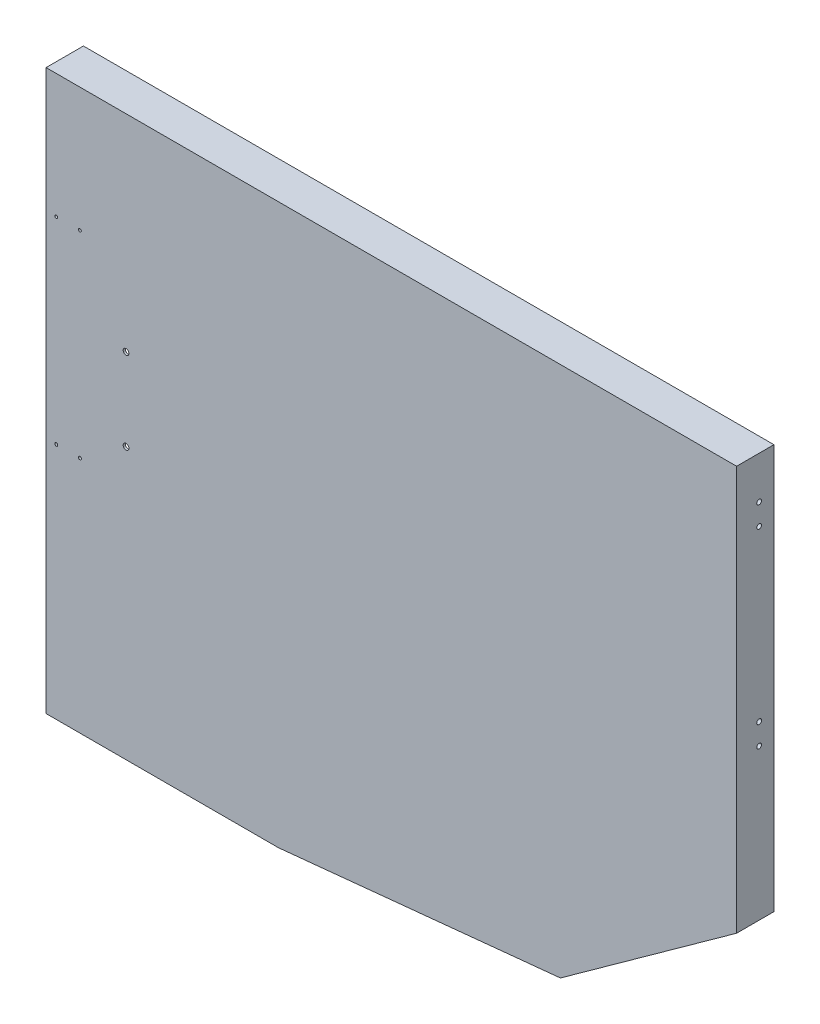
SolidWorks part; units mm, degrees
ref_plane "前视基准面" through (0, 0, 0) normal (0, 0, 1) x (1, 0, 0)
ref_plane "上视基准面" through (0, 0, 0) normal (0, 1, 0) x (1, 0, 0)
ref_plane "右视基准面" through (0, 0, 0) normal (1, 0, 0) x (0, 0, -1)
other "Configuration Table"
sketch "草图1" plane through (0, 0, 0) normal (0, 0, 1) x (1, 0, 0)
  line L0 (550, 375) -> (550, -199)
  line L5 (550, -199) -> (300, -379)
  line L6 (-100, -419) -> (-610, -470) construction
  line L7 (-610, -470) -> (-610, 375) construction
  line L8 (-610, 375) -> (550, 375) construction
  line L10 (-100, -419) -> (300, -379)
  line L11 (-111, 375) -> (550, 375)
  line L12 (-100, -419) -> (-430, -419)
  line L13 (-111, 375) -> (-430, 375)
  line L14 (-430, 375) -> (-430, -419)
  dimension "D1" = 1160
  dimension "D2" = 574
  dimension "D3" = 794
  dimension "D4" = 250
  dimension "D5" = 180
  dimension "D7" = 400
  dimension "D8" = 550
  dimension "D9" = 375
  dimension "D10" = 330
extrude "拉伸-薄壁1" add sketch "草图1" along normal blind 53 thin
sketch "草图2" plane through (0, 0, 53) normal (0, 0, -1) x (-1, 0, 0)
  line L0 (100, -419) -> (430, -419)
  line L3 (430, -419) -> (430, 375)
  line L10 (-300, -379) -> (-550, -199) construction
  line L11 (100, -419) -> (-300, -379) construction
  line L13 (-550, 375) -> (430, 375) construction
  line L14 (-550, -199) -> (-550, 375) construction
  line L15 (-300, -379) -> (-550, -199)
  line L16 (100, -419) -> (-300, -379)
  line L18 (-550, 375) -> (430, 375)
  line L19 (-550, -199) -> (-550, 375)
extrude "凸台-拉伸1" add sketch "草图2" along normal blind 3
sketch "草图3" plane through (0, 0, 50) normal (0, 0, -1) x (-1, 0, 0)
  line L0 (-550, 375) -> (430, 375) construction
  line L1 (-542, 375) -> (-550, 375)
  line L2 (-542, 375) -> (-542, -199.0633)
  line L3 (-544.8657, -199) -> (-550, -199)
  line L4 (-550, 375) -> (-550, -199)
  line L5 (-300, -379) -> (-550, -199) construction
  line L6 (-550, -199) -> (-550, 375) construction
  line L7 (-544.8657, -199) -> (-542, -201.0633)
  line L8 (-298.9004, -376.095) -> (-547, -197.4633) construction
  line L9 (-542, -201.0633) -> (-542, -199.0633)
  line L10 (-298.9004, -376.095) -> (-547, -197.4633) construction
  dimension "D1" = 8
  dimension "D2" = 2
extrude "凸台-拉伸2" add sketch "草图3" along normal up to surface (50 mm away) up to face at (73.3333, -111, 0)
sketch "草图4" plane through (0, 372, 0) normal (0, -1, 0) x (1, 0, 0)
  line L0 (492, 50) -> (542, 8)
  line L1 (542, 50) -> (-427, 50) construction
  line L2 (542, 0) -> (542, 50) construction
  line L3 (542, 0) -> (-427, 0) construction
  dimension "D1" = 8
  dimension "D2" = 50
extrude "拉伸-薄壁3" add sketch "草图4" along normal up to surface (609.0633 mm away) thin thin type one direction reverse wall 2
sketch "草图5" plane through (0, 0, 53) normal (0, 0, 1) x (1, 0, 0)
  circle A0 centre (-316.5, 82.25) radius 4.1
  circle A1 centre (-316.5, -34.25) radius 4.1
  dimension "D1" = 8.2
extrude "切除-拉伸1" cut sketch "草图5" against normal up to next
sketch "草图8" plane through (550, 0, 0) normal (1, 0, 0) x (0, 0, -1)
  point P0 (-21, 315)
  point P3 (-21, 285)
  point P6 (-21, 45)
  point P9 (-21, 15)
hole_wizard "M8 螺纹孔1" positions "草图8" profile "草图7" tap size "M8" standard "GB"
cosmetic thread "孔螺纹线1" parameters "D2"=8
cosmetic thread "孔螺纹线2" parameters "D2"=8
cosmetic thread "孔螺纹线3" parameters "D2"=8
cosmetic thread "孔螺纹线4" parameters "D2"=8
sketch "草图7" plane through (550, 315, 21) normal (0, 1, 0) x (0, 0, -1)
  line L0 (0, 0) -> (0, 8)
  line L1 (0, 8) -> (3.4, 8)
  line L2 (3.4, 8) -> (3.4, 0)
  line L5 (3.4, 0) -> (0, 0)
  line L11 (0, -6.35) -> (0, 107.95) construction
  dimension "通孔螺纹孔钻头直径" = 6.8
  dimension "通孔螺纹孔钻头深度" = 8
sketch "草图11" plane through (0, 0, 53) normal (0, 0, 1) x (1, 0, 0)
  line L0 (-430, 375) -> (-430, -419) construction
  point P0 (-415.5147, 199)
  point P3 (-382.0147, 199)
  point P6 (-415.5147, -81)
  point P9 (-382.0147, -81)
  point P17 (-415.5147, -81)
  point P20 (-382.0147, -81)
  point P26 (-415.5147, 199)
  point P29 (-382.0147, 199)
  dimension "D1" = 14.4853
hole_wizard "M5 螺纹孔1" positions "草图11" profile "草图10" tap size "M5" standard "GB"
sketch "草图10" plane through (-415.5147, 199, 53) normal (1, 0, 0) x (0, -1, 0)
  line L0 (0, 0) -> (0, 15.2618)
  line L1 (0, 15.2618) -> (2.1, 14)
  line L2 (2.1, 14) -> (2.1, 0)
  line L5 (2.1, 0) -> (0, 0)
  line L10 (0, 15.2618) -> (-2.1, 14) construction
  line L11 (0, -6.35) -> (0, 107.95) construction
  dimension "螺纹孔钻头直径" = 4.2
  dimension "螺纹孔钻头深度" = 14
  dimension "导头角度" = 118
cosmetic thread "孔螺纹线5" parameters "D1"=10, "D2"=5
cosmetic thread "孔螺纹线6" parameters "D1"=10, "D2"=5
cosmetic thread "孔螺纹线7" parameters "D1"=10, "D2"=5
cosmetic thread "孔螺纹线8" parameters "D1"=10, "D2"=5
